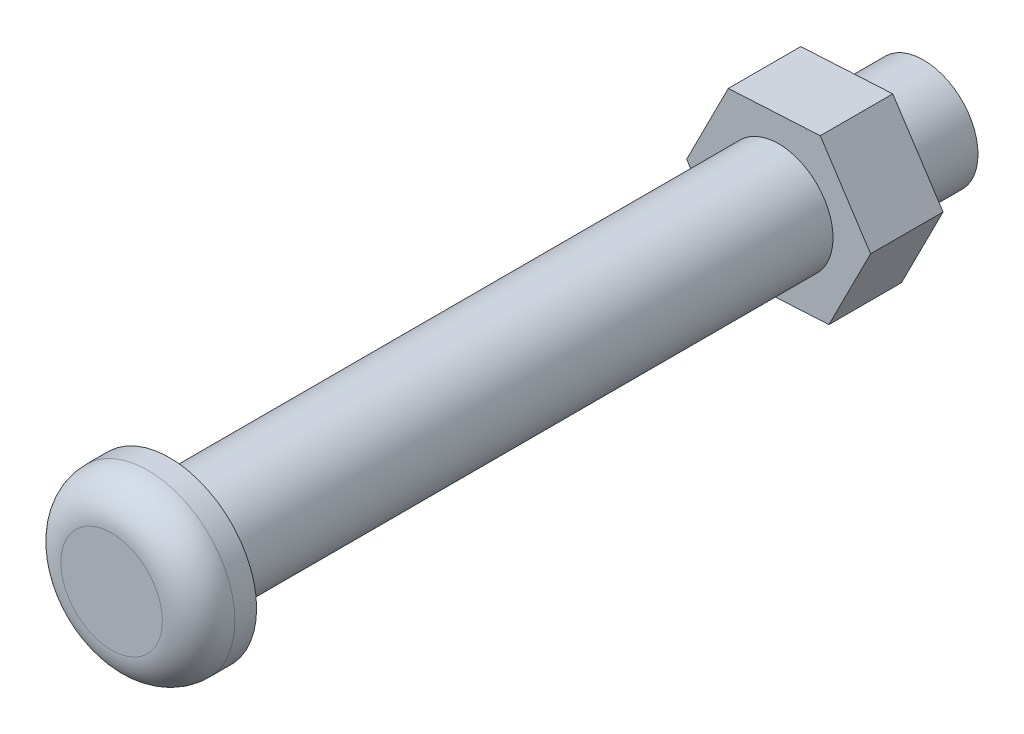
SolidWorks part; units mm, degrees
ref_plane "Front" through (0, 0, 0) normal (0, 0, 1) x (1, 0, 0)
ref_plane "Top" through (0, 0, 0) normal (0, 1, 0) x (1, 0, 0)
ref_plane "Right" through (0, 0, 0) normal (1, 0, 0) x (0, 0, -1)
sketch "Sketch1" plane through (0, 0, 0) normal (0, 0, 1) x (1, 0, 0)
  circle A0 centre (-34.925, -76.2) radius 4.7625
  dimension "D1" = 9.525
extrude "Boss-Extrude1" add sketch "Sketch1" against normal offset from surface (66.04 mm away) 12.7
sketch "Sketch2" plane through (0, 0, 0) normal (0, 0, 1) x (1, 0, 0)
  circle A0 centre (-34.925, -76.2) radius 7.62
  dimension "D1" = 15.24
extrude "Boss-Extrude2" add sketch "Sketch2" along normal blind 5.08
fillet "Fillet1" radius 3.175 1 edges at (-27.305, -76.2, 5.08)
sketch "Sketch3" plane through (0, 0, -53.34) normal (0, 0, -1) x (-1, 0, 0)
  line L1 (39.3312, -69.4444) -> (31.2776, -69.0063)
  line L2 (31.2776, -69.0063) -> (26.8713, -75.7619)
  line L3 (26.8713, -75.7619) -> (30.5188, -82.9556)
  line L4 (30.5188, -82.9556) -> (38.5724, -83.3937)
  line L5 (38.5724, -83.3937) -> (42.9787, -76.6381)
  line L6 (42.9787, -76.6381) -> (39.3312, -69.4444)
  circle A0 centre (34.925, -76.2) radius 4.7625
  circle A1 centre (34.925, -76.2) radius 6.985 construction
  dimension "D1" = 13.97
extrude "Boss-Extrude3" add sketch "Sketch3" along normal blind 6.35 separate body
